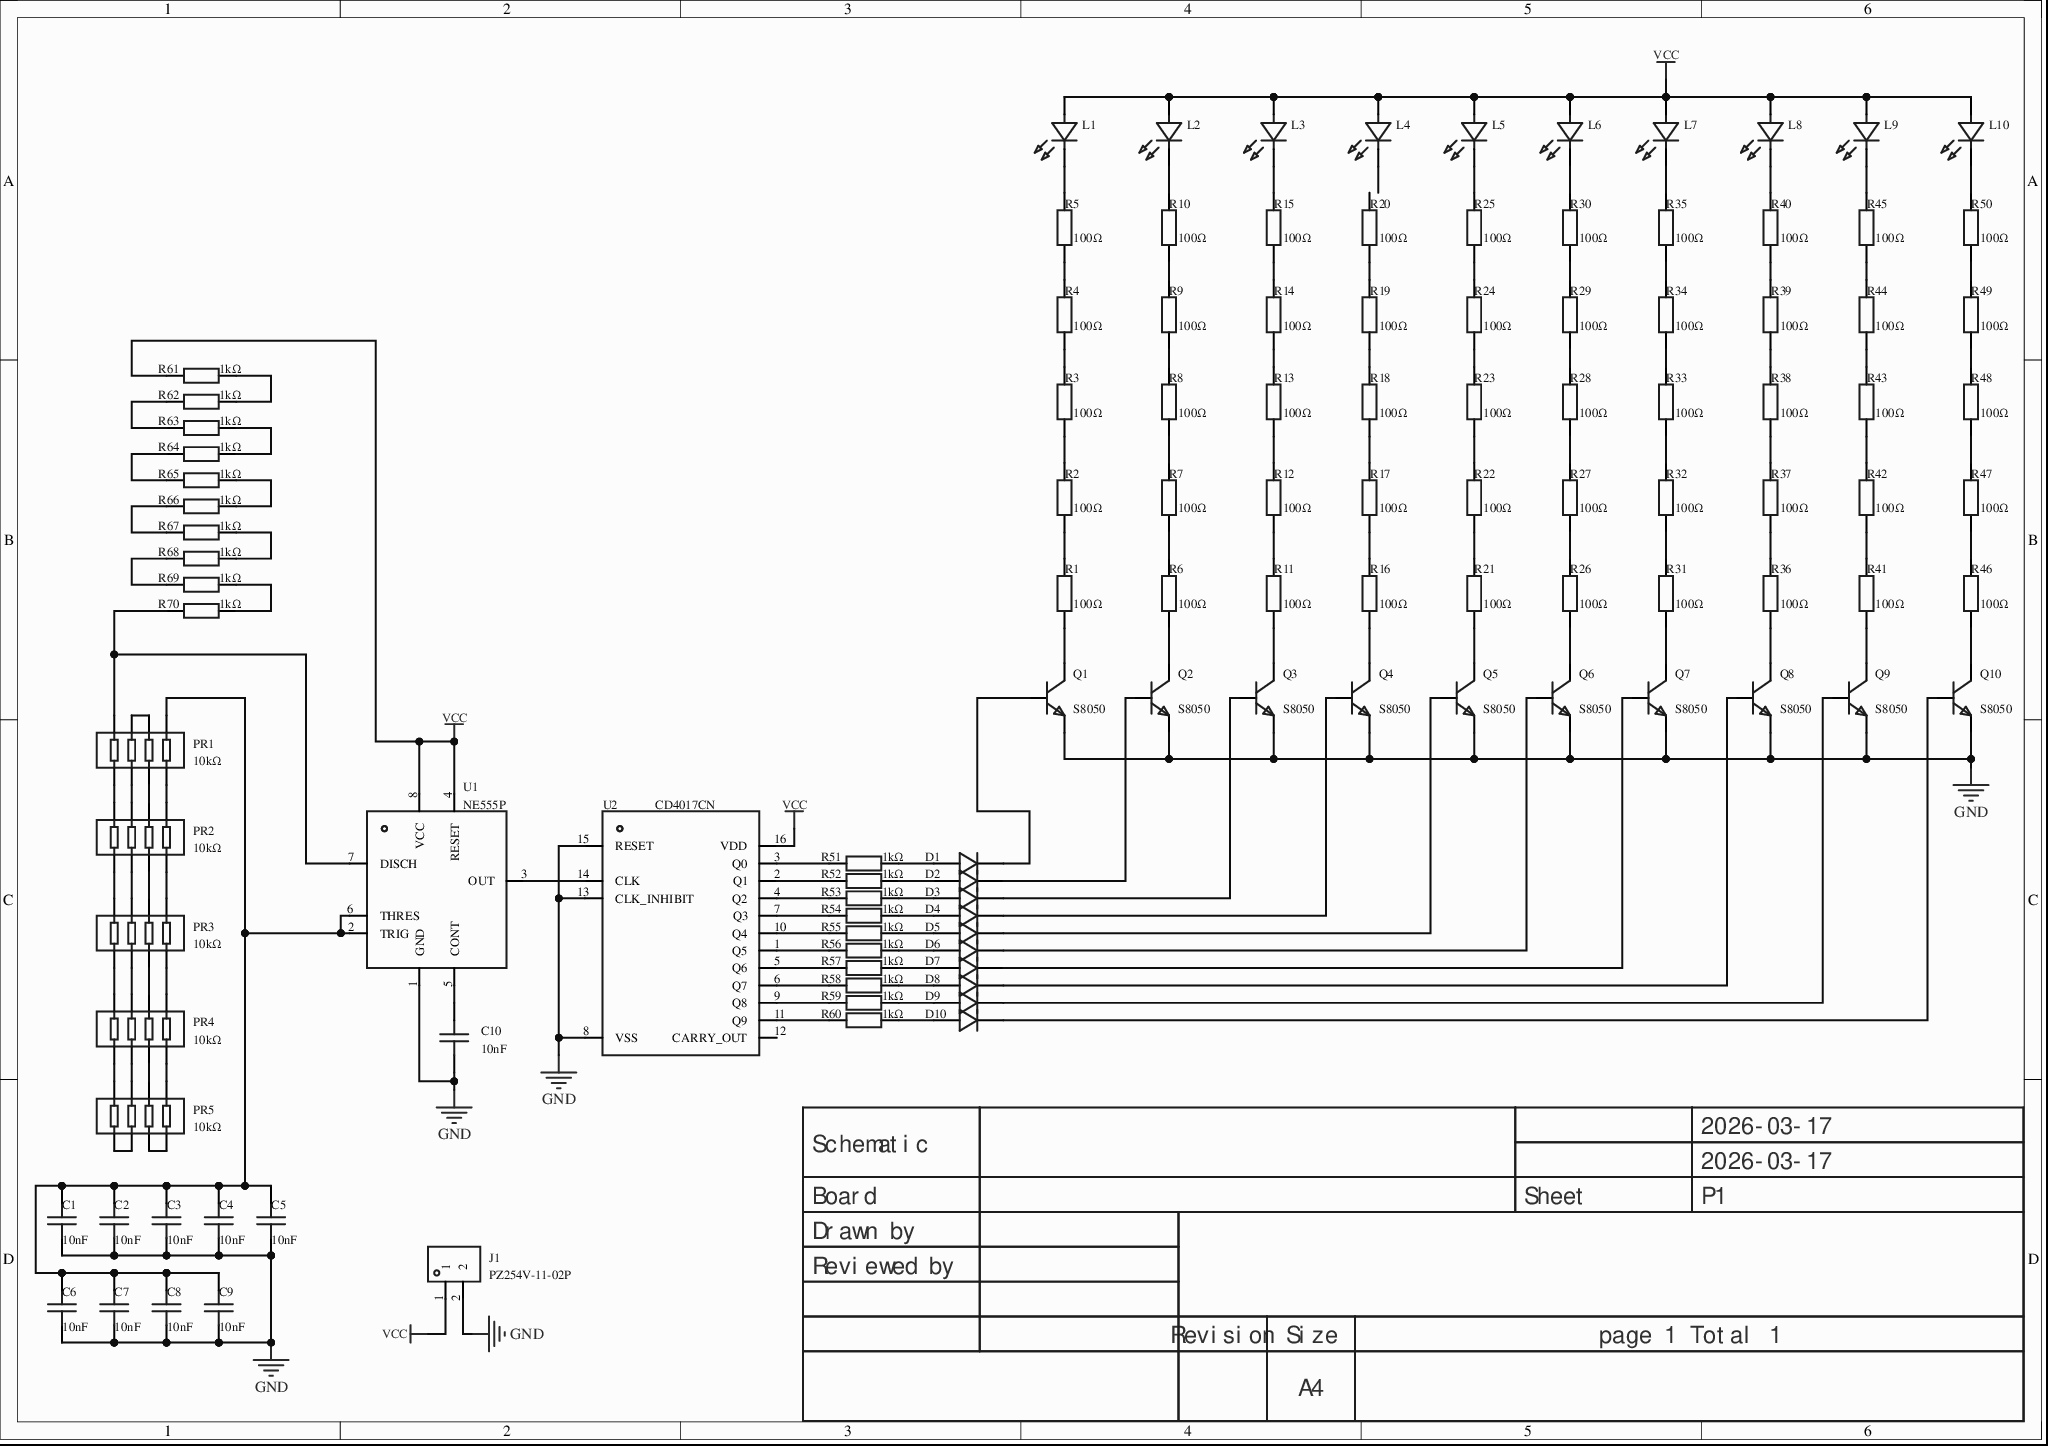
[diagram p0: MISC52150-3.schdoc]
# Altium project MISC52150-2.PrjPcb
1 sheet, 118 parts. Net scope: global (net labels, ports and power ports of the same name join across sheets).
Board file: MISC52150.pcbdoc

## Sheet MISC52150-3.schdoc
size 297 x 209 mm; Version: V1.0; @Project Name: MISC52150; @Page Count: 1; @Update Date: 2026-03-17; @Create Date: 2026-03-17; @Schematic Name: MISC52150; @Page No: 1; @Board Name: MISC52150; @Create Time: 14:32:28; @Update Time: 14:38:12; Size: A4

### Parts
C1  10nF  [CAP-TH_L8.0-W2.8-P5.08-D0.6]
C2  10nF  [CAP-TH_L8.0-W2.8-P5.08-D0.6]
C3  10nF  [CAP-TH_L8.0-W2.8-P5.08-D0.6]
C4  10nF  [CAP-TH_L8.0-W2.8-P5.08-D0.6]
C5  10nF  [CAP-TH_L8.0-W2.8-P5.08-D0.6]
C6  10nF  [CAP-TH_L8.0-W2.8-P5.08-D0.6]
C7  10nF  [CAP-TH_L8.0-W2.8-P5.08-D0.6]
C8  10nF  [CAP-TH_L8.0-W2.8-P5.08-D0.6]
C9  10nF  [CAP-TH_L8.0-W2.8-P5.08-D0.6]
C10  10nF  [CAP-TH_L8.0-W2.8-P5.08-D0.6]
D1  1N4148TR  [DO-35_BD2.0-L4.2-P8.20-D0.5-RD]  (value not drawn)
D2  1N4148TR  [DO-35_BD2.0-L4.2-P8.20-D0.5-RD]  (value not drawn)
D3  1N4148TR  [DO-35_BD2.0-L4.2-P8.20-D0.5-RD]  (value not drawn)
D4  1N4148TR  [DO-35_BD2.0-L4.2-P8.20-D0.5-RD]  (value not drawn)
D5  1N4148TR  [DO-35_BD2.0-L4.2-P8.20-D0.5-RD]  (value not drawn)
D6  1N4148TR  [DO-35_BD2.0-L4.2-P8.20-D0.5-RD]  (value not drawn)
D7  1N4148TR  [DO-35_BD2.0-L4.2-P8.20-D0.5-RD]  (value not drawn)
D8  1N4148TR  [DO-35_BD2.0-L4.2-P8.20-D0.5-RD]  (value not drawn)
D9  1N4148TR  [DO-35_BD2.0-L4.2-P8.20-D0.5-RD]  (value not drawn)
D10  1N4148TR  [DO-35_BD2.0-L4.2-P8.20-D0.5-RD]  (value not drawn)
J1  PZ254V-11-02P  [HDR-TH_2P-P2.54-V-M]
L1  XL-502SURD  [LED-TH_BD5.9-P2.54-RD_RED]  (value not drawn)
L2  XL-502SURD  [LED-TH_BD5.9-P2.54-RD_RED]  (value not drawn)
L3  XL-502SURD  [LED-TH_BD5.9-P2.54-RD_RED]  (value not drawn)
L4  XL-502SURD  [LED-TH_BD5.9-P2.54-RD_RED]  (value not drawn)
L5  XL-502SURD  [LED-TH_BD5.9-P2.54-RD_RED]  (value not drawn)
L6  XL-502SURD  [LED-TH_BD5.9-P2.54-RD_RED]  (value not drawn)
L7  XL-502SURD  [LED-TH_BD5.9-P2.54-RD_RED]  (value not drawn)
L8  XL-502SURD  [LED-TH_BD5.9-P2.54-RD_RED]  (value not drawn)
L9  XL-502SURD  [LED-TH_BD5.9-P2.54-RD_RED]  (value not drawn)
L10  XL-502SURD  [LED-TH_BD5.9-P2.54-RD_RED]  (value not drawn)
PR1  10kΩ  [RES-ARRAY-TH_8P-L20.3-W2.5-P2.54]
PR2  10kΩ  [RES-ARRAY-TH_8P-L20.3-W2.5-P2.54]
PR3  10kΩ  [RES-ARRAY-TH_8P-L20.3-W2.5-P2.54]
PR4  10kΩ  [RES-ARRAY-TH_8P-L20.3-W2.5-P2.54]
PR5  10kΩ  [RES-ARRAY-TH_8P-L20.3-W2.5-P2.54]
Q1  S8050  [TO-92-3_L4.5-W3.5-P1.27-L]
Q2  S8050  [TO-92-3_L4.5-W3.5-P1.27-L]
Q3  S8050  [TO-92-3_L4.5-W3.5-P1.27-L]
Q4  S8050  [TO-92-3_L4.5-W3.5-P1.27-L]
Q5  S8050  [TO-92-3_L4.5-W3.5-P1.27-L]
Q6  S8050  [TO-92-3_L4.5-W3.5-P1.27-L]
Q7  S8050  [TO-92-3_L4.5-W3.5-P1.27-L]
Q8  S8050  [TO-92-3_L4.5-W3.5-P1.27-L]
Q9  S8050  [TO-92-3_L4.5-W3.5-P1.27-L]
Q10  S8050  [TO-92-3_L4.5-W3.5-P1.27-L]
R1  100Ω  [RES-TH_BD2.2-L6.5-P10.50-D0.6]
R2  100Ω  [RES-TH_BD2.2-L6.5-P10.50-D0.6]
R3  100Ω  [RES-TH_BD2.2-L6.5-P10.50-D0.6]
R4  100Ω  [RES-TH_BD2.2-L6.5-P10.50-D0.6]
R5  100Ω  [RES-TH_BD2.2-L6.5-P10.50-D0.6]
R6  100Ω  [RES-TH_BD2.2-L6.5-P10.50-D0.6]
R7  100Ω  [RES-TH_BD2.2-L6.5-P10.50-D0.6]
R8  100Ω  [RES-TH_BD2.2-L6.5-P10.50-D0.6]
R9  100Ω  [RES-TH_BD2.2-L6.5-P10.50-D0.6]
R10  100Ω  [RES-TH_BD2.2-L6.5-P10.50-D0.6]
R11  100Ω  [RES-TH_BD2.2-L6.5-P10.50-D0.6]
R12  100Ω  [RES-TH_BD2.2-L6.5-P10.50-D0.6]
R13  100Ω  [RES-TH_BD2.2-L6.5-P10.50-D0.6]
R14  100Ω  [RES-TH_BD2.2-L6.5-P10.50-D0.6]
R15  100Ω  [RES-TH_BD2.2-L6.5-P10.50-D0.6]
R16  100Ω  [RES-TH_BD2.2-L6.5-P10.50-D0.6]
R17  100Ω  [RES-TH_BD2.2-L6.5-P10.50-D0.6]
R18  100Ω  [RES-TH_BD2.2-L6.5-P10.50-D0.6]
R19  100Ω  [RES-TH_BD2.2-L6.5-P10.50-D0.6]
R20  100Ω  [RES-TH_BD2.2-L6.5-P10.50-D0.6]
R21  100Ω  [RES-TH_BD2.2-L6.5-P10.50-D0.6]
R22  100Ω  [RES-TH_BD2.2-L6.5-P10.50-D0.6]
R23  100Ω  [RES-TH_BD2.2-L6.5-P10.50-D0.6]
R24  100Ω  [RES-TH_BD2.2-L6.5-P10.50-D0.6]
R25  100Ω  [RES-TH_BD2.2-L6.5-P10.50-D0.6]
R26  100Ω  [RES-TH_BD2.2-L6.5-P10.50-D0.6]
R27  100Ω  [RES-TH_BD2.2-L6.5-P10.50-D0.6]
R28  100Ω  [RES-TH_BD2.2-L6.5-P10.50-D0.6]
R29  100Ω  [RES-TH_BD2.2-L6.5-P10.50-D0.6]
R30  100Ω  [RES-TH_BD2.2-L6.5-P10.50-D0.6]
R31  100Ω  [RES-TH_BD2.2-L6.5-P10.50-D0.6]
R32  100Ω  [RES-TH_BD2.2-L6.5-P10.50-D0.6]
R33  100Ω  [RES-TH_BD2.2-L6.5-P10.50-D0.6]
R34  100Ω  [RES-TH_BD2.2-L6.5-P10.50-D0.6]
R35  100Ω  [RES-TH_BD2.2-L6.5-P10.50-D0.6]
R36  100Ω  [RES-TH_BD2.2-L6.5-P10.50-D0.6]
R37  100Ω  [RES-TH_BD2.2-L6.5-P10.50-D0.6]
R38  100Ω  [RES-TH_BD2.2-L6.5-P10.50-D0.6]
R39  100Ω  [RES-TH_BD2.2-L6.5-P10.50-D0.6]
R40  100Ω  [RES-TH_BD2.2-L6.5-P10.50-D0.6]
R41  100Ω  [RES-TH_BD2.2-L6.5-P10.50-D0.6]
R42  100Ω  [RES-TH_BD2.2-L6.5-P10.50-D0.6]
R43  100Ω  [RES-TH_BD2.2-L6.5-P10.50-D0.6]
R44  100Ω  [RES-TH_BD2.2-L6.5-P10.50-D0.6]
R45  100Ω  [RES-TH_BD2.2-L6.5-P10.50-D0.6]
R46  100Ω  [RES-TH_BD2.2-L6.5-P10.50-D0.6]
R47  100Ω  [RES-TH_BD2.2-L6.5-P10.50-D0.6]
R48  100Ω  [RES-TH_BD2.2-L6.5-P10.50-D0.6]
R49  100Ω  [RES-TH_BD2.2-L6.5-P10.50-D0.6]
R50  100Ω  [RES-TH_BD2.2-L6.5-P10.50-D0.6]
R51  1kΩ  [RES-TH_BD2.5-L6.5-P10.50-D0.6]
R52  1kΩ  [RES-TH_BD2.5-L6.5-P10.50-D0.6]
R53  1kΩ  [RES-TH_BD2.5-L6.5-P10.50-D0.6]
R54  1kΩ  [RES-TH_BD2.5-L6.5-P10.50-D0.6]
R55  1kΩ  [RES-TH_BD2.5-L6.5-P10.50-D0.6]
R56  1kΩ  [RES-TH_BD2.5-L6.5-P10.50-D0.6]
R57  1kΩ  [RES-TH_BD2.5-L6.5-P10.50-D0.6]
R58  1kΩ  [RES-TH_BD2.5-L6.5-P10.50-D0.6]
R59  1kΩ  [RES-TH_BD2.5-L6.5-P10.50-D0.6]
R60  1kΩ  [RES-TH_BD2.5-L6.5-P10.50-D0.6]
R61  1kΩ  [RES-TH_BD2.5-L6.5-P10.50-D0.6]
R62  1kΩ  [RES-TH_BD2.5-L6.5-P10.50-D0.6]
R63  1kΩ  [RES-TH_BD2.5-L6.5-P10.50-D0.6]
R64  1kΩ  [RES-TH_BD2.5-L6.5-P10.50-D0.6]
R65  1kΩ  [RES-TH_BD2.5-L6.5-P10.50-D0.6]
R66  1kΩ  [RES-TH_BD2.5-L6.5-P10.50-D0.6]
R67  1kΩ  [RES-TH_BD2.5-L6.5-P10.50-D0.6]
R68  1kΩ  [RES-TH_BD2.5-L6.5-P10.50-D0.6]
R69  1kΩ  [RES-TH_BD2.5-L6.5-P10.50-D0.6]
R70  1kΩ  [RES-TH_BD2.5-L6.5-P10.50-D0.6]
U1  NE555P  [DIP-8_L9.8-W6.6-P2.54-LS7.6-BL]
U2  CD4017CN  [PDIP-16_L19.3-W6.4-P2.54-LS7.94-BL]

### Nets
GND: C1.1 C2.1 C3.1 C4.1 C5.1 C6.1 C7.1 C8.1 C9.1 C10.1 J1.2 Q1.1(E) Q2.1(E) Q3.1(E) Q4.1(E) Q5.1(E) Q6.1(E) Q7.1(E) Q8.1(E) Q9.1(E) Q10.1(E) U1.1(GND) U2.8(VSS) U2.13(CLK_INHIBIT) U2.15(RESET)
VCC: J1.1 L1.2(A) L2.2(A) L3.2(A) L4.2(A) L5.2(A) L6.2(A) L7.2(A) L8.2(A) L9.2(A) L10.2(A) R61.1 U1.4(RESET) U1.8(VCC) U2.16(VDD)
NetC1_2: C1.2 C2.2 C3.2 C4.2 C5.2 C6.2 C7.2 C8.2 C9.2 PR1.5 U1.2(TRIG) U1.6(THRES)
NetC10_2: C10.2 U1.5(CONT)
NetD1_1: D1.1(C) Q1.2(B)
NetD1_2: D1.2(A) R51.2
NetD2_1: D2.1(C) Q2.2(B)
NetD2_2: D2.2(A) R52.2
NetD3_1: D3.1(C) Q3.2(B)
NetD3_2: D3.2(A) R53.2
NetD4_1: D4.1(C) Q4.2(B)
NetD4_2: D4.2(A) R54.2
NetD5_1: D5.1(C) Q5.2(B)
NetD5_2: D5.2(A) R55.2
NetD6_1: D6.1(C) Q6.2(B)
NetD6_2: D6.2(A) R56.2
NetD7_1: D7.1(C) Q7.2(B)
NetD7_2: D7.2(A) R57.2
NetD8_1: D8.1(C) Q8.2(B)
NetD8_2: D8.2(A) R58.2
NetD9_1: D9.1(C) Q9.2(B)
NetD9_2: D9.2(A) R59.2
NetD10_1: D10.1(C) Q10.2(B)
NetD10_2: D10.2(A) R60.2
NetL1_1: L1.1(K) R5.2
NetL2_1: L2.1(K) R10.2
NetL3_1: L3.1(K) R15.2
NetL5_1: L5.1(K) R25.2
NetL6_1: L6.1(K) R30.2
NetL7_1: L7.1(K) R35.2
NetL8_1: L8.1(K) R40.2
NetL9_1: L9.1(K) R45.2
NetL10_1: L10.1(K) R50.2
NetPR1_1: PR1.1 PR2.8
NetPR1_2: PR1.2 PR2.7
NetPR1_3: PR1.3 PR2.6
NetPR1_4: PR1.4 PR2.5
NetPR1_6: PR1.6 PR1.7
NetPR1_8: PR1.8 R70.1 U1.7(DISCH)
NetPR2_1: PR2.1 PR3.8
NetPR2_2: PR2.2 PR3.7
NetPR2_3: PR2.3 PR3.6
NetPR2_4: PR2.4 PR3.5
NetPR3_1: PR3.1 PR4.8
NetPR3_2: PR3.2 PR4.7
NetPR3_3: PR3.3 PR4.6
NetPR3_4: PR3.4 PR4.5
NetPR4_1: PR4.1 PR5.8
NetPR4_2: PR4.2 PR5.7
NetPR4_3: PR4.3 PR5.6
NetPR4_4: PR4.4 PR5.5
NetPR5_1: PR5.1 PR5.2
NetPR5_3: PR5.3 PR5.4
NetQ1_3: Q1.3(C) R1.1
NetQ2_3: Q2.3(C) R6.1
NetQ3_3: Q3.3(C) R11.1
NetQ4_3: Q4.3(C) R16.1
NetQ5_3: Q5.3(C) R21.1
NetQ6_3: Q6.3(C) R26.1
NetQ7_3: Q7.3(C) R31.1
NetQ8_3: Q8.3(C) R36.1
NetQ9_3: Q9.3(C) R41.1
NetQ10_3: Q10.3(C) R46.1
NetR1_2: R1.2 R2.1
NetR2_2: R2.2 R3.1
NetR3_2: R3.2 R4.1
NetR4_2: R4.2 R5.1
NetR6_2: R6.2 R7.1
NetR7_2: R7.2 R8.1
NetR8_2: R8.2 R9.1
NetR9_2: R9.2 R10.1
NetR11_2: R11.2 R12.1
NetR12_2: R12.2 R13.1
NetR13_2: R13.2 R14.1
NetR14_2: R14.2 R15.1
NetR16_2: R16.2 R17.1
NetR17_2: R17.2 R18.1
NetR18_2: R18.2 R19.1
NetR19_2: R19.2 R20.1
NetR21_2: R21.2 R22.1
NetR22_2: R22.2 R23.1
NetR23_2: R23.2 R24.1
NetR24_2: R24.2 R25.1
NetR26_2: R26.2 R27.1
NetR27_2: R27.2 R28.1
NetR28_2: R28.2 R29.1
NetR29_2: R29.2 R30.1
NetR31_2: R31.2 R32.1
NetR32_2: R32.2 R33.1
NetR33_2: R33.2 R34.1
NetR34_2: R34.2 R35.1
NetR36_2: R36.2 R37.1
NetR37_2: R37.2 R38.1
NetR38_2: R38.2 R39.1
NetR39_2: R39.2 R40.1
NetR41_2: R41.2 R42.1
NetR42_2: R42.2 R43.1
NetR43_2: R43.2 R44.1
NetR44_2: R44.2 R45.1
NetR46_2: R46.2 R47.1
NetR47_2: R47.2 R48.1
NetR48_2: R48.2 R49.1
NetR49_2: R49.2 R50.1
NetR51_1: R51.1 U2.3(Q0)
NetR52_1: R52.1 U2.2(Q1)
NetR53_1: R53.1 U2.4(Q2)
NetR54_1: R54.1 U2.7(Q3)
NetR55_1: R55.1 U2.10(Q4)
NetR56_1: R56.1 U2.1(Q5)
NetR57_1: R57.1 U2.5(Q6)
NetR58_1: R58.1 U2.6(Q7)
NetR59_1: R59.1 U2.9(Q8)
NetR60_1: R60.1 U2.11(Q9)
NetR61_2: R61.2 R62.2
NetR62_1: R62.1 R63.1
NetR63_2: R63.2 R64.2
NetR64_1: R64.1 R65.1
NetR65_2: R65.2 R66.2
NetR66_1: R66.1 R67.1
NetR67_2: R67.2 R68.2
NetR68_1: R68.1 R69.1
NetR69_2: R69.2 R70.2
NetU1_3: U1.3(OUT) U2.14(CLK)

Not connected (* = marked no-connect by the designer): L4 1(K); R20 2; U2 12(CARRY_OUT)

### Notes on the sheet
- 2026-03-17
- Schematic
- Board
- Sheet
- P1
- Drawn by
- Reviewed by
- Revision
- Size
- A4
- page 1 Total 1

### Library data of the parts
C1-C10 = CC3A103MC1IEF48C30MF: Capacitance: 10nF; tolerance: ±20%; rated voltage: 1kV; temperature coefficient: Y5V;; Manufacturer: Dersonic(德尔创); AddInBom: yes; ModelId: 68e147d5135c46d1ae59b8b7da6d9a28; ModelTransform: 314.45,110.236,0,0,0,0,0,0,-196.85; Pin Spacing: 5.08mm; Body Thickness: 2.8mm; Symbol: CC3A103MC1IEF48C30MF; Device: CC3A103MC1IEF48C30MF; LCSC Part Name: 10nF ±20% 1kV; SupplierPart: C263209; ManufacturerPart: CC3A103MC1IEF48C30MF; Supplier Footprint: 插件,P=5.08mm; JLCPCB Part Class: Extended library; Datasheet: https://example.com/datasheet/CC3A103MC1IEF48C30MF/254325.html; Supplier: LCSC; ConvertToPcb: yes; FootprintName: CAP-TH_L8.0-W2.8-P5.08-D0.6; ModelName: CAP-TH_L8.0-W2.8-P5.08-D0.6; Value: 10nF; Tolerance: ±20%; Voltage Rating: 1kV; Temperature Coefficient: Y5V; Diameter: 8mm
D1-D10 = 1N4148TR_C84410: Diode configuration: -; forward voltage (Vf): 1V@10mA; DC reverse voltage (Vr): 100V; rectified current: 200mA; reverse recovery time (Trr): 4ns;; Manufacturer: onsemi(安森美); AddInBom: yes; ModelId: 6e6fa891745c42b796728c269d94cdcf; ModelName: DO-35_D1.9-L3.9-P8.2; ModelTransform: 342.519,74.82103,0,0,0,0,-0.197,1.181,-137.795; Pd - Power Dissipation: 500mW; Reverse Leakage Current (Ir): 5uA@75V; Operating Junction Temperature Range: -55℃~+175℃@(Tj); Non-Repetitive Peak Forward Surge Current: 4A; Symbol: 1N4148TR; Device: 1N4148TR_C84410; LCSC Part Name: 1N4148TR; SupplierPart: C84410; ManufacturerPart: 1N4148TR; Supplier Footprint: DO-35; JLCPCB Part Class: Extended library; Datasheet: https://example.com/datasheet/1N4148TR/85580.html; Supplier: LCSC; ConvertToPcb: yes; FootprintName: DO-35_BD2.0-L4.2-P8.20-D0.5-RD; Diode Configuration: -; Voltage - Forward(Vf@If): 1V@10mA; Voltage - DC Reverse(Vr): 100V; Current - Rectified: 200mA; Reverse Recovery Time (trr): 4ns
J1 = PZ254V-11-02P: Pin structure: 1x2P; pitch: 2.54mm; row spacing: -; round/square pin: square pin; mounting: through-hole; rows: single row; total pins: 2P; rated current: 3A; rated voltage: 250V; mating pin length: 6mm; housing height: 2.5mm; tail pin length: 3mm; contact material: brass; contact plating: -; operating temperature: -40℃~+105℃; color: black;; Manufacturer: XFCN(兴飞); AddInBom: yes; ModelId: e35305ec3aa84b66b849f914b715e73f; ModelName: HDR2.54-M-LI-1X2P; ModelTransform: 200,100,0,0,0,0,0,0,-118.11; Symbol: PZ254V-11-02P; Device: PZ254V-11-02P; LCSC Part Name: 1x2P 间距:2.54mm 方针 直插; SupplierPart: C492401; ManufacturerPart: PZ254V-11-02P; Supplier Footprint: 插件,P=2.54mm; JLCPCB Part Class: Extended library; Datasheet: https://example.com/datasheet/PZ254V-11-02P/502957.html; Supplier: LCSC; ConvertToPcb: yes; FootprintName: HDR-TH_2P-P2.54-V-M; Pin Structure: 1x2P; Pitch: 2.54mm; Row Spacing: -; Circluar Pins/Square Pins: Square pin; Mounting Type: Through-hole; Number of Rows: Single row; Number of Pins: 2P; Current Rating: 3A; Voltage Rating (Max): 250V; Length of Mating Pin: 6mm; Insulation Height: 2.5mm; Length of End Connection Pin: 3mm; Contact Material: Brass; Contact Plating: -; Operating Temperature: -40℃~+105℃; Color: Black
L1-L10 = XL-502SURD: Lamp holder type: 5mm round lamp holder; luminous color: red; forward voltage (Vf): 2.4V; power: 70mW; forward current: 20mA; wavelength: 615nm~625nm; diode configuration: -; lens color: red lens; color temperature: -; luminous intensity: 300mcd; viewing angle: 35°; tape and reel: -; operating temperature: -25℃~+85℃;; Manufacturer: XINGLIGHT(成兴光); AddInBom: yes; ModelId: fe9cea1bdf7642cd8d9a5077ed0e2b58; ModelTransform: 211.96686,228.01584,0,0,0,0,7.874,0,-137.795; Peak Wavelength: 654nm; Symbol: XL-502SURD; Device: XL-502SURD; LCSC Part Name: 5mm圆形灯头 红色; SupplierPart: C2895492; ManufacturerPart: XL-502SURD; Supplier Footprint: 插件,D=5mm; JLCPCB Part Class: Extended library; Datasheet: https://example.com/datasheet/XL-502SURD/3136207.html; Supplier: LCSC; ConvertToPcb: yes; FootprintName: LED-TH_BD5.9-P2.54-RD_RED; ModelName: LED-TH_BD5.9-P2.54-RD_RED; Lamp Holder Type: 5mm round lamp holder; Illumination Color: Red; Voltage - Forward(Vf): 2.4V; Power(Watts): 70mW; Forward Current: 20mA; Wavelength - Dominant: 615nm~625nm; Diode Configuration: -; Lens Color: Red lens; Color Temperature: -; Luminous Intensity: 300mcd; Viewing Angle: 35°; Mounting Style: -; Operating Temperature: -25℃~+85℃
PR1-PR5 = 4608X-102-103LF: Number of resistors: 4; resistance: 10kΩ; tolerance: ±2%; power per element: 300mW; temperature coefficient: ±100ppm/℃;; Manufacturer: BOURNS; AddInBom: yes; ModelId: 1fcaf8e202754517bf5022a866f874ea; ModelTransform: 798.02982,98.031,0,0,0,0,0,0,-133.858; Number of Resistors: 4; Symbol: 4608X-102-103LF; Device: 4608X-102-103LF; LCSC Part Name: 10kΩ ±2%; SupplierPart: C840662; ManufacturerPart: 4608X-102-103LF; Supplier Footprint: SIP-8; JLCPCB Part Class: Extended library; Datasheet: https://example.com/datasheet/4608X-102-103LF/897114.html; Supplier: LCSC; ConvertToPcb: yes; FootprintName: RES-ARRAY-TH_8P-L20.3-W2.5-P2.54; ModelName: RES-ARRAY-TH_8P-L20.3-W2.5-P2.54; Value: 10kΩ; Tolerance: ±2%; Power(Watts): 300mW; Temperature Coefficient: ±100ppm/℃; Number of Pins: 8
Q1-Q10 = S8050_C2931492: Transistor type: NPN; collector current (Ic): 500mA; collector-emitter breakdown voltage (Vceo): 25V; power dissipation (Pd): 625mW; DC current gain (hFE): 160@50mA,1V;; Manufacturer: JSMSEMI(杰盛微); AddInBom: yes; ModelId: 45fa6cddef3743c6aacf8db740a3bc4c; ModelTransform: 177.165,137.795,0,0,0,0,0,29.528,-98.425; Transition frequency(fT): 150MHz; Current - Collector Cutoff: 100nA; Vce Saturation(VCE(sat)): 600mV@500mA,50mA; Emitter-Base Voltage(Vebo): 5V; Symbol: S8050_C2931492; Device: S8050_C2931492; LCSC Part Name: NPN 电流:500mA 电压:25V; SupplierPart: C2931492; ManufacturerPart: S8050; Supplier Footprint: TO-92; JLCPCB Part Class: Extended library; Datasheet: https://example.com/datasheet/S8050/3272796.html; Supplier: LCSC; ConvertToPcb: yes; FootprintName: TO-92-3_L4.5-W3.5-P1.27-L; ModelName: TO-92-3_L4.5-W3.5-P1.27-L; type: NPN; Current - Collector(Ic): 500mA; Collector - Emitter Voltage VCEO: 25V; Pd - Power Dissipation: 625mW; DC Current Gain: 160@50mA,1V
R1-R50 = MFR0W4F1000A50: Resistor type: metal film resistor; resistance: 100Ω; tolerance: ±1%; power: 250mW; temperature coefficient: ±50ppm/℃;; Manufacturer: UNI-ROYAL(厚声); AddInBom: yes; ModelId: 259c3103781c424fb695c8049f0a17f3; ModelTransform: 437.007,91.18383,0,0,0,0,0,0,-137.795; Voltage-Supply(Max): 250V; Symbol: MFR0W4F1000A50; Device: MFR0W4F1000A50; LCSC Part Name: 100Ω ±1% 250mW 金属膜电阻 铜脚，圆柱状直插; SupplierPart: C57438; ManufacturerPart: MFR0W4F1000A50; Supplier Footprint: 插件,D2.2xL6.5mm; JLCPCB Part Class: Extended library; Datasheet: https://example.com/upload/public/pdf/source/20191012/C436293_8820AA14BC71FA35E551C06C441482A0.pdf; Supplier: LCSC; ConvertToPcb: yes; FootprintName: RES-TH_BD2.2-L6.5-P10.50-D0.6; ModelName: RES-TH_BD2.2-L6.5-P10.50-D0.6; Type: Metal film resistor; Value: 100Ω; Tolerance: ±1%; Power(Watts): 250mW; Temperature Coefficient: ±50ppm/℃
R51-R70 = MFR0W4F1001A50: Resistor type: metal film resistor; resistance: 1kΩ; tolerance: ±1%; power: 250mW; temperature coefficient: ±50ppm/℃;; Manufacturer: UNI-ROYAL(厚声); AddInBom: yes; ModelId: 8e6c7ee8323443d1ab8f0504b6353c8c; ModelName: RES-TH_D2.3-L6.5-P10.50; ModelTransform: 431.1015,91.3384,0,0,0,0,0.197,0,-137.795; Voltage-Supply(Max): 250V; Symbol: MFR0W4F1001A50; Device: MFR0W4F1001A50; LCSC Part Name: 1kΩ ±1% 250mW 金属膜电阻 铜脚，圆柱状直插; SupplierPart: C57435; ManufacturerPart: MFR0W4F1001A50; Supplier Footprint: 插件,D2.2xL6.5mm; JLCPCB Part Class: Extended library; Datasheet: https://example.com/upload/public/pdf/source/20191012/C436293_8820AA14BC71FA35E551C06C441482A0.pdf; Supplier: LCSC; ConvertToPcb: yes; FootprintName: RES-TH_BD2.5-L6.5-P10.50-D0.6; Type: Metal film resistor; Value: 1kΩ; Tolerance: ±1%; Power(Watts): 250mW; Temperature Coefficient: ±50ppm/℃
U1 = NE555P: These devices are precision timing circuits that generate accurate time delays or oscillation. In delay or monostable mode, the timing interval is set by a single external resistor and capacitor network. In astable mode, frequency and duty cycle are controlled separately by two external resistors and one external capacitor.; Manufacturer: TI(德州仪器); AddInBom: yes; ModelId: db2af726fcec488f8bf8e467aca974b3; ModelName: DIP-8_L9.8-W6.6-H3.5-LS7.62-P2.54; ModelTransform: 385.826,311.8104,0,0,0,0,-1.693,0,-137.795; Symbol: NE555P; Device: NE555P; LCSC Part Name: NE555P; SupplierPart: C46749; ManufacturerPart: NE555P; Supplier Footprint: DIP-8; JLCPCB Part Class: Extended Part; Supplier: LCSC; ConvertToPcb: yes; FootprintName: DIP-8_L9.8-W6.6-P2.54-LS7.6-BL
U2 = CD4017CN: CD4017BE upgraded replacement, sample recommended; 5-stage Johnson decade counter; Manufacturer: HGSEMI(华冠); AddInBom: yes; ModelId: 96ff5d01b3074dd183bcbc4cd00a63de; ModelTransform: 759.841,322.44,0,0,0,0,0,0,-137.795; Symbol: CD4017CN; Device: CD4017CN; LCSC Part Name: CD4017CN; SupplierPart: C20613262; ManufacturerPart: CD4017CN; Supplier Footprint: DIP-16; JLCPCB Part Class: Extended library; Datasheet: https://example.com/upload/public/pdf/source/20240202/A11F5FEC5EC92025B33B6A151300674C.pdf; Supplier: LCSC; ConvertToPcb: yes; FootprintName: PDIP-16_L19.3-W6.4-P2.54-LS7.94-BL; ModelName: PDIP-16_L19.3-W6.4-P2.54-LS7.94-BL